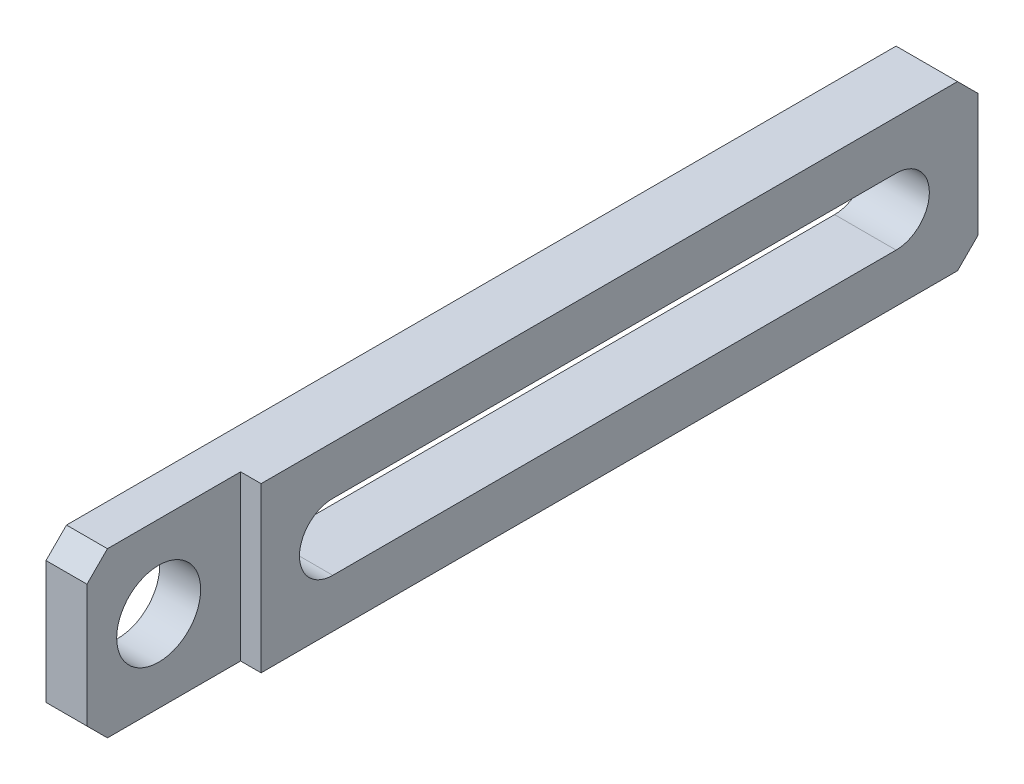
from build123d import *

# Parameters (mm, degrees)
SKETCH1_W                  = 85
SKETCH1_H                  = 16
EXTRUDE1_DEPTH             = 6
F_8_2_8_2_DIAMETER_HOLE1_D = 8.2
CHAMFER1_SIZE              = 2
SKETCH5_W                  = 15
SKETCH5_H                  = 16
CUT_EXTRUDE1_DEPTH         = 2


with BuildPart() as part:
    # Sketch1 → Extrude1 (new body)
    with BuildSketch(Plane(origin=(0, 0, 0), x_dir=(0, 0, -1), z_dir=(1, 0, 0))):
        with Locations((42.5, -8)):
            Rectangle(SKETCH1_W, SKETCH1_H)
        with BuildLine():
            Line((22, -4.75), (77, -4.75))
            ThreePointArc((77, -4.75), (80.25, -8), (77, -11.25))
            Line((77, -11.25), (22, -11.25))
            ThreePointArc((22, -11.25), (18.75, -8), (22, -4.75))
        make_face(mode=Mode.SUBTRACT)
    extrude(amount=EXTRUDE1_DEPTH)

    # Ø8.2 (8.2) Diameter Hole1 (through all)
    with Locations(Plane(origin=(6, 0, 0), x_dir=(0, 0, -1), z_dir=(1, 0, 0))):
        with Locations((7, -8)):
            Hole(F_8_2_8_2_DIAMETER_HOLE1_D / 2)

    # Chamfer1
    chamfer1_edges = [part.edges().sort_by_distance(p)[0] for p in [
        (3, 0, 0),
        (3, 0, -85),
        (3, -16, -85),
        (3, -16, 0),
    ]]
    chamfer(chamfer1_edges, length=CHAMFER1_SIZE)

    # Sketch5 → Cut-Extrude1 (cut)
    with BuildSketch(Plane(origin=(6, 0, 0), x_dir=(0, 0, -1), z_dir=(1, 0, 0))):
        with Locations((7.5, -8)):
            Rectangle(SKETCH5_W, SKETCH5_H)
    extrude(amount=-CUT_EXTRUDE1_DEPTH, mode=Mode.SUBTRACT)


solid = part.part
